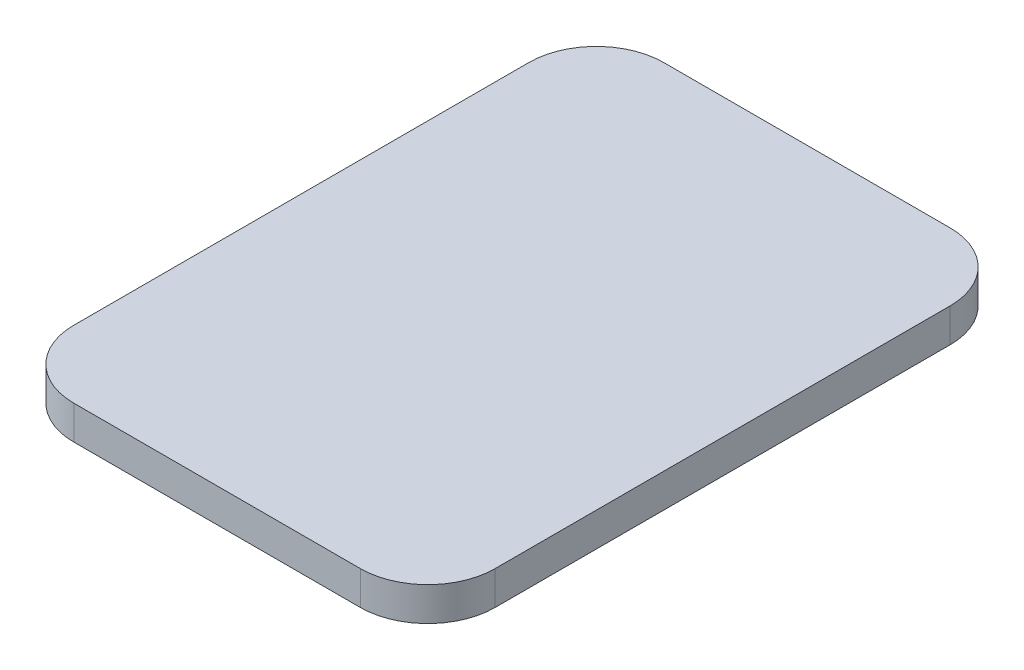
from build123d import *

# Parameters (mm, degrees)
BOSS_EXTRU_1_DEPTH = 2


with BuildPart() as part:
    # Sketch1 → Boss.-Extru.1 (new body)
    with BuildSketch(Plane(origin=(0, 0, 0), x_dir=(1, 0, 0), z_dir=(0, 1, 0))):
        with BuildLine():
            Line((8.5, 17.5), (-8.5, 17.5))
            ThreePointArc((-8.5, 17.5), (-11.328427125, 16.328427125), (-12.5, 13.5))
            Line((-12.5, 13.5), (-12.5, -13.5))
            ThreePointArc((-12.5, -13.5), (-11.328427125, -16.328427125), (-8.5, -17.5))
            Line((-8.5, -17.5), (8.5, -17.5))
            ThreePointArc((8.5, -17.5), (11.328427125, -16.328427125), (12.5, -13.5))
            Line((12.5, -13.5), (12.5, 13.5))
            ThreePointArc((12.5, 13.5), (11.328427125, 16.328427125), (8.5, 17.5))
        make_face()
    extrude(amount=BOSS_EXTRU_1_DEPTH)


solid = part.part
